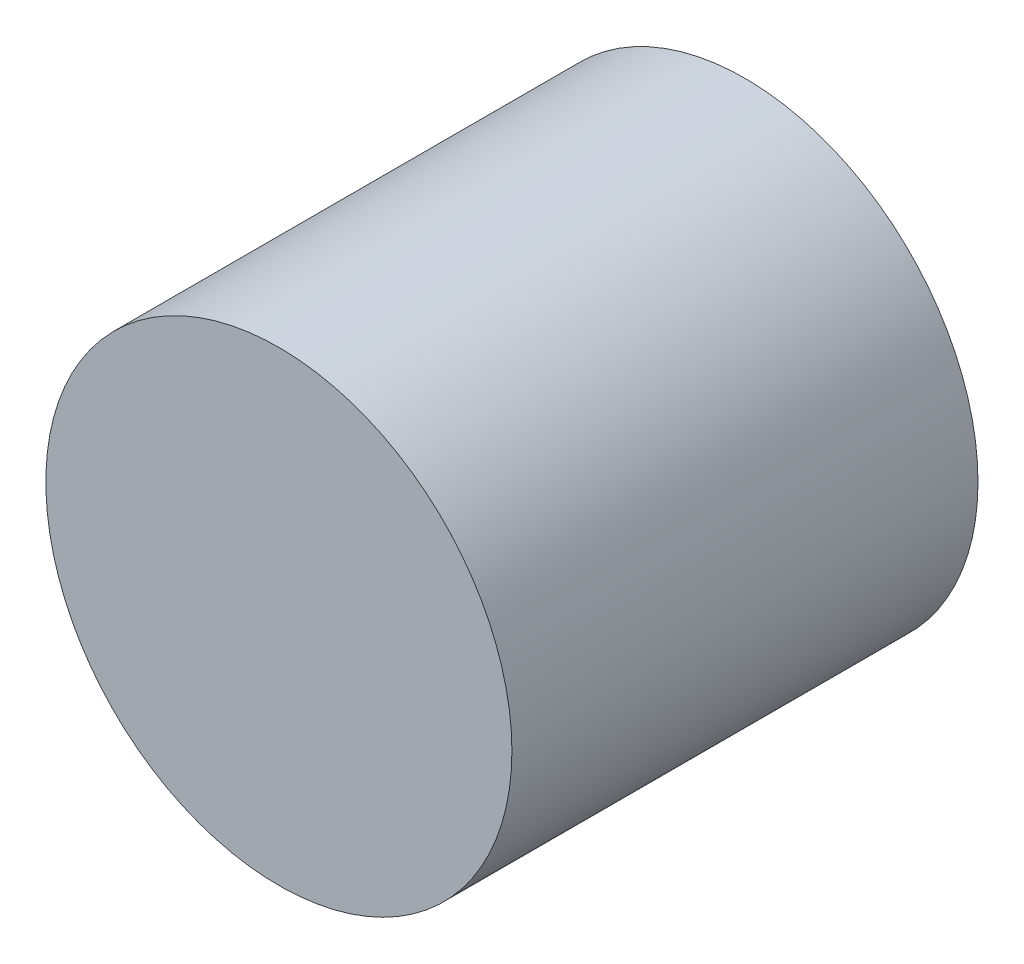
from build123d import *

# Parameters (mm, degrees)
SKETCH1_R           = 9.5
BOSS_EXTRUDE1_DEPTH = 19


with BuildPart() as part:
    # Sketch1 → Boss-Extrude1 (new body)
    with BuildSketch(Plane.XY):
        Circle(SKETCH1_R)
    extrude(amount=BOSS_EXTRUDE1_DEPTH)


solid = part.part
